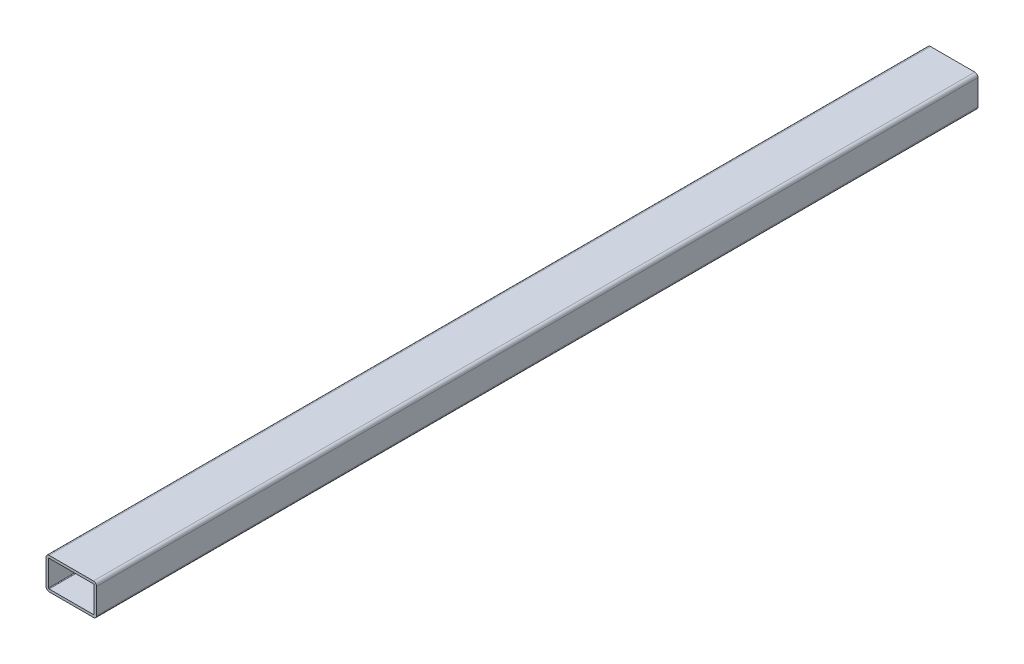
from build123d import *

# Parameters (mm, degrees)
BOSS_EXTRUDE1_DEPTH = 1393
SHELL1_T            = -4


with BuildPart() as part:
    # Sketch1 → Boss-Extrude1 (new body)
    with BuildSketch(Plane.XY):
        with BuildLine():
            Line((35, 25), (-35, 25))
            ThreePointArc((-35, 25), (-38.535533906, 23.535533906), (-40, 20))
            Line((-40, 20), (-40, -20))
            ThreePointArc((-40, -20), (-38.535533906, -23.535533906), (-35, -25))
            Line((-35, -25), (35, -25))
            ThreePointArc((35, -25), (38.535533906, -23.535533906), (40, -20))
            Line((40, -20), (40, 20))
            ThreePointArc((40, 20), (38.535533906, 23.535533906), (35, 25))
        make_face()
    extrude(amount=BOSS_EXTRUDE1_DEPTH)

    # Shell1
    shell1_openings = [part.faces().sort_by_distance(p)[0] for p in [
        (0, 0, 1393),
        (0, 0, 0),
    ]]
    offset(amount=SHELL1_T, openings=shell1_openings, kind=Kind.INTERSECTION)


solid = part.part
